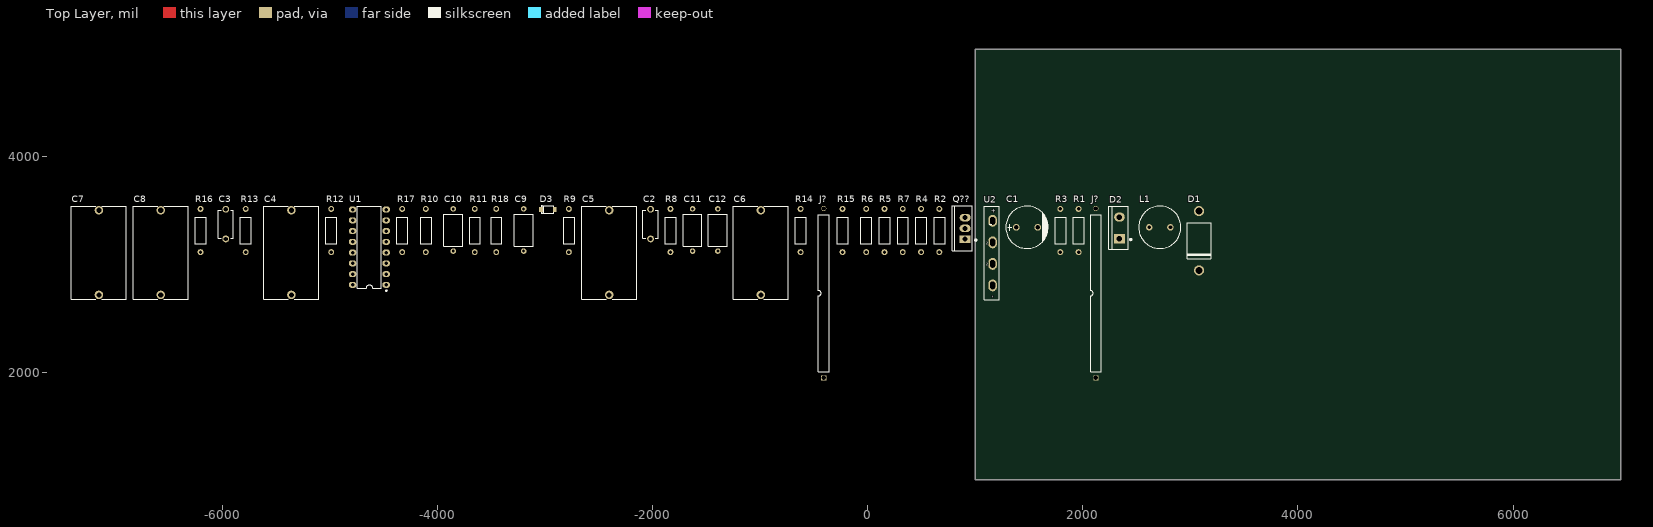
[diagram p0: Top Layer view]
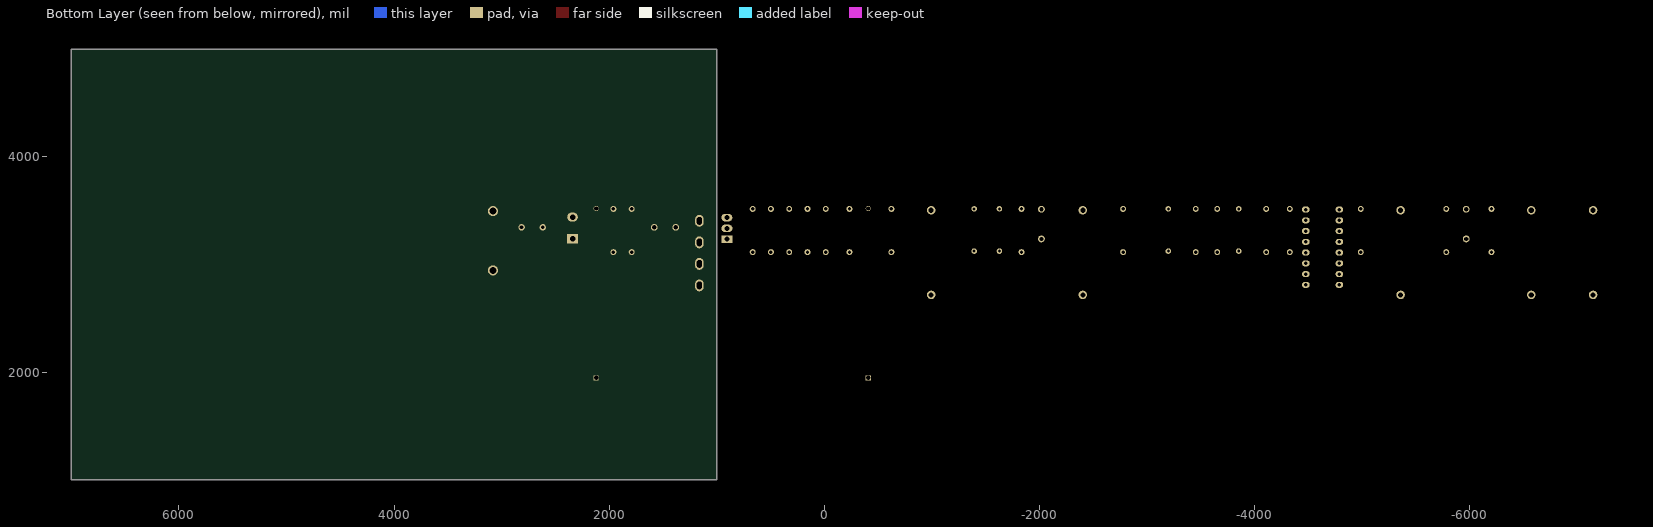
[diagram p1: Bottom Layer view, seen from below]
# Altium PCB MISC82375-15.PcbDoc
Units mil, origin at the board's own origin, x right, y up, seen from the top; angles counter-clockwise.
Board outline 6000 x 4000 mil, 2 copper layers (Top Layer, Bottom Layer); 39 components, 26 nets, 95 pads, 0 vias.
Unrouted connection lines stored in the file: 18.

## Layer stack, top to bottom (the 12.6 mil dielectric is the usual default, probably not edited)
Top Solder: solder mask 0.4, Solder Resist, Dk 3.5
Top Layer: signal copper 1.4
Dielectric 1: dielectric 12.6, FR-4, Dk 4.8
Bottom Layer: signal copper 1.4
Bottom Solder: solder mask 0.4, Solder Resist, Dk 3.5

## Board outline
1000,1000 7000,1000 7000,5000 1000,5000

## Design rules (kind name [scope] priority, off if disabled: settings)
Clearance [All] p1: gap=10 ignorepadtopadclearanceinfootprint=FALSE except(0: Arc-Hole Track-Hole SMDPad-Hole THPad-Hole Via-Hole Fill-Hole Poly-Hole Region-Hole Text-Hole)
PolygonConnect [All] p1: connectstyle=Relief reliefconductorwidth=10 reliefentries=4 polygonreliefangle="90 Angle" airgapwidth=10
RoutingVias [All] p1: holewidth=28 width=50 viastyle="Through Hole" minholewidth=28 minwidth=50 maxholewidth=28 maxwidth=50
SolderMaskExpansion [All] p1: expansion=4 istentingtop=FALSE
Width [All] p1: maxlimit=10 minlimit=10 preferedwidth=10
30 further rules are at their usual default settings.

## Components (designator, comment, footprint, x,y, rotation, side; value= is the part's Value field where it differs from the comment)
C1 "LKME1402A101MF" CAP-TH_BD10.0-P5.00-D1.0-FD 1480,3345.58 r0 top value=100uF
C2 "KJKF222M2FF7035A075E" CAP-TH_L6.5-W3.5-P7.50-D1.0 -2020,3375.58 r90 top value=2.2nF
C3 "KJKF222M2FF7035A075E" CAP-TH_L6.5-W3.5-P7.50-D1.0 -5970,3375.58 r90 top value=2.2nF
C4 "CBB21-400V/255JP20" CAP-TH_L22.0-W12.5-P20.00-D0.7-FD -5360,3110.58 r90 top value=2.5uF
C5 "CBB21-400V/255JP20" CAP-TH_L22.0-W12.5-P20.00-D0.7-FD -2405,3110.58 r90 top value=2.5uF
C6 "CBB21-400V/255JP20" CAP-TH_L22.0-W12.5-P20.00-D0.7-FD -995,3110.58 r90 top value=2.5uF
C7 "CBB21-400V/255JP20" CAP-TH_L22.0-W12.5-P20.00-D0.7-FD -7150,3110.58 r90 top value=2.5uF
C8 "CBB21-400V/255JP20" CAP-TH_L22.0-W12.5-P20.00-D0.7-FD -6575,3110.58 r90 top value=2.5uF
C9 "KY1102M400VAC70Y10093" CAP-TH_L7.5-W4.5-P10.00-D0.6 -3200,3320.58 r90 top value=1nF
C10 "KY1102M400VAC70Y10093" CAP-TH_L7.5-W4.5-P10.00-D0.6 -3855,3320.58 r90 top value=1nF
C11 "KY1102M400VAC70Y10093" CAP-TH_L7.5-W4.5-P10.00-D0.6 -1630,3320.58 r90 top value=1nF
C12 "KY1102M400VAC70Y10093" CAP-TH_L7.5-W4.5-P10.00-D0.6 -1395,3320.58 r90 top value=1nF
D1 "1N5406_C5338388" DO-27_BD5.2-L8.9-P12.90-D1.5-RD 3080,3220.58 r90 top
D2 "GC3D10060A" TO-220-2_L10.2-W4.5-P5.08-L-A 2340,3340.58 r90 top
D3 "BZT52C8V2_C19077406" SOD-123_L2.7-W1.6-LS3.7-RD -2975,3510.58 r0 top
J? "2" "DIP2 - duplicate" -410,1945.58 r90 top
J? "2" "DIP2 - duplicate" 2120,1945.58 r90 top
L1 "XR8*10-101K-L" IND-TH_BD10.0-P5.00-D0.6 2715,3345.58 r0 top value=100uH
Q?? "IRF530NPBF" TO-220-3_L10.0-W4.5-P2.54-L 905,3335.58 r90 top
R1 "MF1/4W-100K±1%-OT26" RES-TH_BD2.7-L6.2-P10.20-D0.4 1960,3315.58 r90 top value=100kΩ
R2 "MF1/4W-100K±1%-OT26" RES-TH_BD2.7-L6.2-P10.20-D0.4 665,3315.58 r90 top value=100kΩ
R3 "MF1/4W-100K±1%-OT26" RES-TH_BD2.7-L6.2-P10.20-D0.4 1790,3315.58 r90 top value=100kΩ
R4 "MF1/4W-100K±1%-OT26" RES-TH_BD2.7-L6.2-P10.20-D0.4 495,3315.58 r90 top value=100kΩ
R5 "MF1/4W-100K±1%-OT26" RES-TH_BD2.7-L6.2-P10.20-D0.4 155,3315.58 r90 top value=100kΩ
R6 "MF1/4W-100K±1%-OT26" RES-TH_BD2.7-L6.2-P10.20-D0.4 -15,3315.58 r90 top value=100kΩ
R7 "MF1/4W-100K±1%-OT26" RES-TH_BD2.7-L6.2-P10.20-D0.4 325,3315.58 r90 top value=100kΩ
R8 "MF1/4W-100K±1%-OT26" RES-TH_BD2.7-L6.2-P10.20-D0.4 -1835,3315.58 r90 top value=100kΩ
R9 "MF1/4W-100K±1%-OT26" RES-TH_BD2.7-L6.2-P10.20-D0.4 -2780,3315.58 r90 top value=100kΩ
R10 "MF1/4W-100K±1%-OT26" RES-TH_BD2.7-L6.2-P10.20-D0.4 -4110,3315.58 r90 top value=100kΩ
R11 "MF1/4W-100K±1%-OT26" RES-TH_BD2.7-L6.2-P10.20-D0.4 -3655,3315.58 r90 top value=100kΩ
R12 "MF1/4W-100K±1%-OT26" RES-TH_BD2.7-L6.2-P10.20-D0.4 -4990,3315.58 r90 top value=100kΩ
R13 "MF1/4W-100K±1%-OT26" RES-TH_BD2.7-L6.2-P10.20-D0.4 -5785,3315.58 r90 top value=100kΩ
R14 "MF1/4W-100K±1%-OT26" RES-TH_BD2.7-L6.2-P10.20-D0.4 -625,3315.58 r90 top value=100kΩ
R15 "MF1/4W-100K±1%-OT26" RES-TH_BD2.7-L6.2-P10.20-D0.4 -235,3315.58 r90 top value=100kΩ
R16 "MF1/4W-100K±1%-OT26" RES-TH_BD2.7-L6.2-P10.20-D0.4 -6205,3315.58 r90 top value=100kΩ
R17 "MF1/4W-100K±1%-OT26" RES-TH_BD2.7-L6.2-P10.20-D0.4 -4330,3315.58 r90 top value=100kΩ
R18 "MF1/4W-100K±1%-OT26" RES-TH_BD2.7-L6.2-P10.20-D0.4 -3455,3315.58 r90 top value=100kΩ
U1 "UC3854N" PDIP-16_L19.3-W6.4-P2.54-LS7.94-BL -4635,3160.58 r90 top
U2 "GBU8K" GBU_4P-L22.0-W3.5-P5.08-GBU4K 1160,3105.58 r90 top

## Footprints (in the part's own frame and the unit in brackets; to place one, negate y for a bottom-side part, rotate by r counter-clockwise, add the part's x,y. Pads: shape width x height; smd on the part's side, far side on the other; paste and mask are expansions set on the pad)
CAP-TH_BD10.0-P5.00-D1.0-FD [mm]
  round 1.6 hole 1: 1(-2.54,0) 2(2.54,0)
  silkscreen extent -5,-5 5.08,5
CAP-TH_L6.5-W3.5-P7.50-D1.0 [mm]
  round 1.6 hole 1: 1(-3.5,0) 2(3.5,0)
  silkscreen extent -3.3,-1.8 3.3,1.8
CAP-TH_L7.5-W4.5-P10.00-D0.6 [mm]
  round 1.3 hole 0.7: 1(-5,0) 2(5,0)
  silkscreen extent -3.8,-2.2 3.7,2.2
CAP-TH_L22.0-W12.5-P20.00-D0.7-FD [mm]
  round 2 hole 1.2: 1(-10,0) 2(10,0)
  silkscreen extent -11,-6.5 11,6.5
"DIP2 - duplicate" [mm]
  rect 1.2x1.2 hole 1: 1(0,0)
  round 1.2 hole 1: 2(40,0)
  silkscreen extent 1.43,-1.25 38.57,1.25
DO-27_BD5.2-L8.9-P12.90-D1.5-RD [mm]
  round 2.4 hole 1.6: 1(-7,0) 2(7,0)
  silkscreen extent -4.3,-2.8 4.3,2.8
GBU_4P-L22.0-W3.5-P5.08-GBU4K [mm]
  oval 2.8x2 hole 1.2 slot 1.8 at 0 deg: 1(-7.62,0) 2(-2.54,0) 3(2.54,0) 4(7.62,0)
  silkscreen extent -11.05,-1.56 11.05,2
IND-TH_BD10.0-P5.00-D0.6 [mm]
  round 1.5 hole 0.9 paste+0 mask+0.05: 1(-2.5,0) 2(2.5,0)
  silkscreen extent -5,-5 5,5
PDIP-16_L19.3-W6.4-P2.54-LS7.94-BL [mm]
  oval 1.44x1.8 hole 0.8: 1(-8.89,-3.97) 2(-6.35,-3.97) 3(-3.81,-3.97) 4(-1.27,-3.97) 5(1.27,-3.97) 6(3.81,-3.97) 7(6.35,-3.97) 8(8.89,-3.97) 9(8.89,3.97) 10(6.35,3.97) 11(3.81,3.97) 12(1.27,3.97) 13(-1.27,3.97) 14(-3.81,3.97) 15(-6.35,3.97) 16(-8.89,3.97)
  silkscreen extent -10.41,-4.17 9.73,2.84
RES-TH_BD2.7-L6.2-P10.20-D0.4 [mm]
  round 1.4 hole 0.8 copper offset 0,0: 1(-5.1,0) 2(5.1,0)
  silkscreen extent -3.1,-1.35 3.1,1.35
SOD-123_L2.7-W1.6-LS3.7-RD [mm]
  rect 0.91x1.22 smd: 1(-1.635,0) 2(1.635,0)
  silkscreen extent -1.6,-1 1.38,1
TO-220-2_L10.2-W4.5-P5.08-L-A [mm]
  rect 2.2x2.5 hole 1.3: 1(-2.54,0)
  oval 2.2x2.5 hole 1.3: 3(2.54,0)
  silkscreen extent -5.1,-2.86 5.1,2.5
TO-220-3_L10.0-W4.5-P2.54-L [mm]
  rect 1.8x2.6 hole 1.2: 1(-2.54,0.005)
  oval 1.8x2.6 hole 1.2: 2(0,0.005)
  oval 1.8x2.6 hole 1.2 copper offset 0,0: 3(2.54,-0.005)
  silkscreen extent -5.3,-2.73 5.3,3.09

## Part data
C1: Equivalent Series Resistance(ESR)=-, JLCPCB Part Class="Extended Part", LCSC Part Name="100uF ±20% 100V", Lifetime @ Temp=10000hrs@105℃, Manufacturer=Ymin(永铭), Rated Voltage=100V, Ripple Current=1.04A@100kHz, Tolerance=±20%
C2: JLCPCB Part Class="Extended Part", LCSC Part Name="2.2nF ±20% 300V 等级:Y2", Manufacturer=KNSCHA(科尼盛), Tolerance=±20%, Voltage(AC)=300V
C3: "0.3uf", JLCPCB Part Class="Extended Part", LCSC Part Name="2.2nF ±20% 300V 等级:Y2", Manufacturer=KNSCHA(科尼盛), Tolerance=±20%, Voltage(AC)=300V
C4 C5 C6 C7 C8: JLCPCB Part Class="Extended Part", LCSC Part Name="2.5uF ±5% 400V", Manufacturer=东通电子, Tolerance=±5%, Voltage Rated=400V
C9 C10 C11 C12: JLCPCB Part Class="Extended Part", LCSC Part Name="1nF ±20% 400V 等级:Y1", Manufacturer=KNSCHA(科尼盛), Tolerance=±20%, Voltage(AC)=400V
D1: Average Rectified Current (Io)=3A, Forward Voltage (Vf@If)=1V@3A, LCSC Part Name="电压:600V 电流:3A", Manufacturer=SUNMATE(森美特), Manufacturer Part=1N5406, Reverse Leakage Current=10uA@600V, Reverse Voltage (Vr)=600V
D2: Average Rectified Current (Io)=30A, Forward Voltage (Vf@If)=1.5V, Manufacturer=SUPSiC(国晶微半导体), Reverse Voltage (Vr)=600V
D3: LCSC Part Name=BZT52C8V2, Manufacturer=宏迦橙, Power Dissipation=500mW, Reverse Leakage Current (Ir)=700nA@5V, Zener Voltage (Nom)=8.2V, Zener Voltage (Range)=7.79V~8.61V
J? J?: library part AC_in
L1: JLCPCB Part Class="Extended Part", LCSC Part Name="100uH ±10% 工字电感", Manufacturer=XR(祥如), Tolerance=±10%
Q??: Continuous Drain Current (Id)=17A, Drain Source On Resistance (RDS(on)@Vgs,Id)=90mΩ@10V,9A, Drain Source Voltage (Vdss)=100V, Gate Threshold Voltage (Vgs(th)@Id)=4V@250uA, Input Capacitance (Ciss@Vds)=920pF@25V, JLCPCB Part Class="Extended Part", LCSC Part Name="N沟道 耐压:100V 电流:17A", Manufacturer=Infineon(英飞凌), Operating Temperature=-55℃~+175℃@(Tj), Power Dissipation (Pd)=70W
R1 R2 R3 R4 R5 R6 R7 R8 R9 R10 R11 R12 R13 R14 R15 R16 R17 R18: JLCPCB Part Class="Extended Part", LCSC Part Name="金属膜电阻 100kΩ ±1% 250mW", Manufacturer=VO(翔胜), Operating Temperature Range=-55℃~+155℃, Overload Voltage (Max)=250V, Power(Watts)=250mW, Temperature Coefficient=±350ppm/℃, Tolerance=±1%
U1: JLCPCB Part Class="Extended Part", Manufacturer=TI(德州仪器), Operating Temperature=0℃~+70℃, Supply Voltage=14.5V~30V, Switching Frequency=200kHz
U2: Average Rectified Current (Io)=8A, Forward Voltage (Vf@If)=1.1V, JLCPCB Part Class="Extended Part", LCSC Part Name="电压:800V 电流:8A", Manufacturer=LRC(乐山无线电), Operating Temperature=-55℃~+150℃@(Tj), Peak Forward Surge Current=175A, Reverse Leakage Current (Ir)=5uA, Reverse Voltage (Vr)=800V

## Nets (pads, with @x,y where several pads share a name; then routed paths per layer and width w, separated by ;. In a path a pad name is that pad's centre, name@x,y a point inside that pad or via, vN(x,y) a via of type N, cw(c..) or ccw(c..) an arc to the next point about the centre after c; other vN are vias at no path point)
GND: C2.1 C3.1 C4.1 C8.2 C9.2 C10.2 C11.1 C12.1 J?.2@-410,3520.39 R13.1 R17.2
NetC1_1: C1.1 D1.1 D2.1 R1.2 R3.2
NetC1_2: C1.2 Q??.3 R2.1 R3.1 R4.2 R7.2
NetC2_2: C2.2 R6.1 R8.2 U1.2
NetC3_2: C3.2 R11.1 R12.1
NetC4_2: C4.2 R12.2 R13.2 U1.8
NetC5_1: C5.1 C6.2 D3.1 U1.3
NetC5_2: C5.2 D3.2 R7.1 R14.1 U1.4
NetC6_1: C6.1 R14.2
NetC7_1: C7.1 R1.1 R2.2 R16.2
NetC7_2: C7.2 R16.1 U1.7
NetC8_1: C8.1 R8.1 R10.2 U1.9
NetC9_1: C9.1 U1.14
NetC10_1: C10.1 U1.13
NetC11_2: C11.2 C12.2 J?.1@-410,1945.58 R18.2 U1.15
NetD1_2: D1.2 L1.1 R9.2 R11.2 U2.4
NetD2_3: D2.3 L1.2 Q??.2
NetJ?_1: J?.1@2120,1945.58 U2.3
NetJ?_2: J?.2@2120,3520.39 U2.2
NetQ??_1: Q??.1 R15.1
NetR4_1: R4.1 R5.2 R6.2 U2.1
NetR5_1: R5.1 U1.5
NetR9_1: R9.1 R10.1 U1.6
NetR15_2: R15.2 U1.16
NetR17_1: R17.1 U1.12
NetR18_1: R18.1 U1.10
pads on no net: U1.1 U1.11